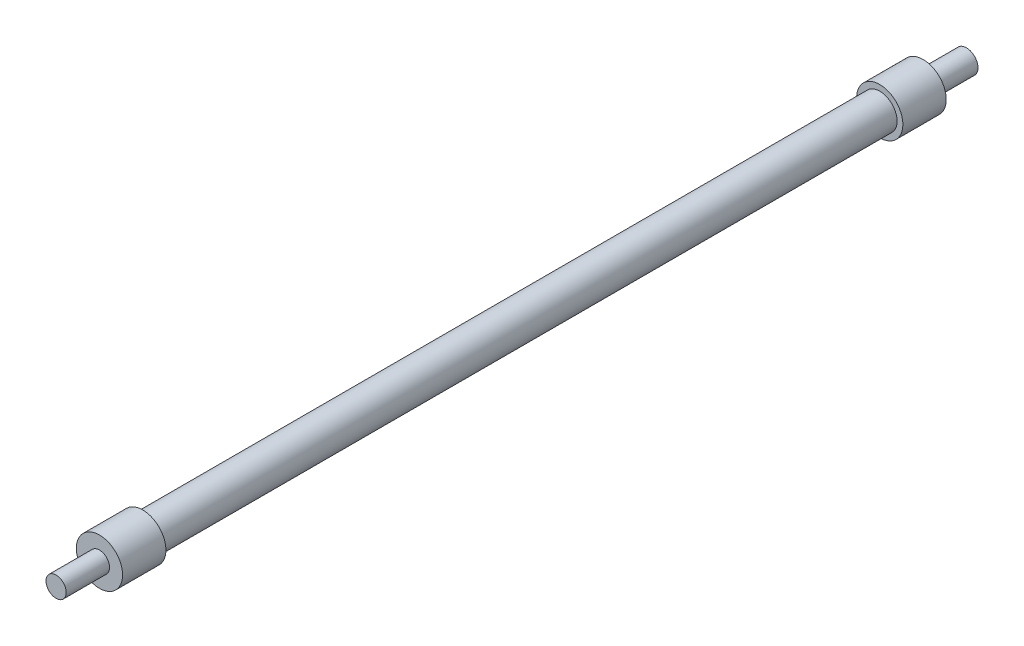
from build123d import *

# Parameters (mm, degrees)
SKETCH_1_R      = 4
EXTRUDE_1_DEPTH = 15
SKETCH_2_R      = 6
EXTRUDE_2_DEPTH = 270
SKETCH_3_R      = 8
EXTRUDE_3_DEPTH = 15
SKETCH_4_R      = 8
EXTRUDE_4_DEPTH = 15
SKETCH_5_R      = 3.5
EXTRUDE_5_DEPTH = 15


with BuildPart() as part:
    # 草图1 → 凸台-拉伸1 (new body)
    with BuildSketch(Plane.XY):
        Circle(SKETCH_1_R)
    extrude(amount=EXTRUDE_1_DEPTH)

    # 草图2 → 凸台-拉伸2 (add)
    with BuildSketch(Plane.XY.offset(15)):
        Circle(SKETCH_2_R)
    extrude(amount=EXTRUDE_2_DEPTH)

    # 草图3 → 凸台-拉伸3 (add)
    with BuildSketch(Plane(origin=(0, 0, 15), x_dir=(-1, 0, 0), z_dir=(0, 0, -1))):
        Circle(SKETCH_3_R)
    extrude(amount=-EXTRUDE_3_DEPTH)

    # 草图4 → 凸台-拉伸4 (add)
    with BuildSketch(Plane.XY.offset(285)):
        with Locations(Location((0, 0, 0), (0, 0, 180))):
            Circle(SKETCH_4_R)
    extrude(amount=EXTRUDE_4_DEPTH)

    # 草图5 → 凸台-拉伸5 (add)
    with BuildSketch(Plane.XY.offset(300)):
        Circle(SKETCH_5_R)
    extrude(amount=EXTRUDE_5_DEPTH)


solid = part.part
